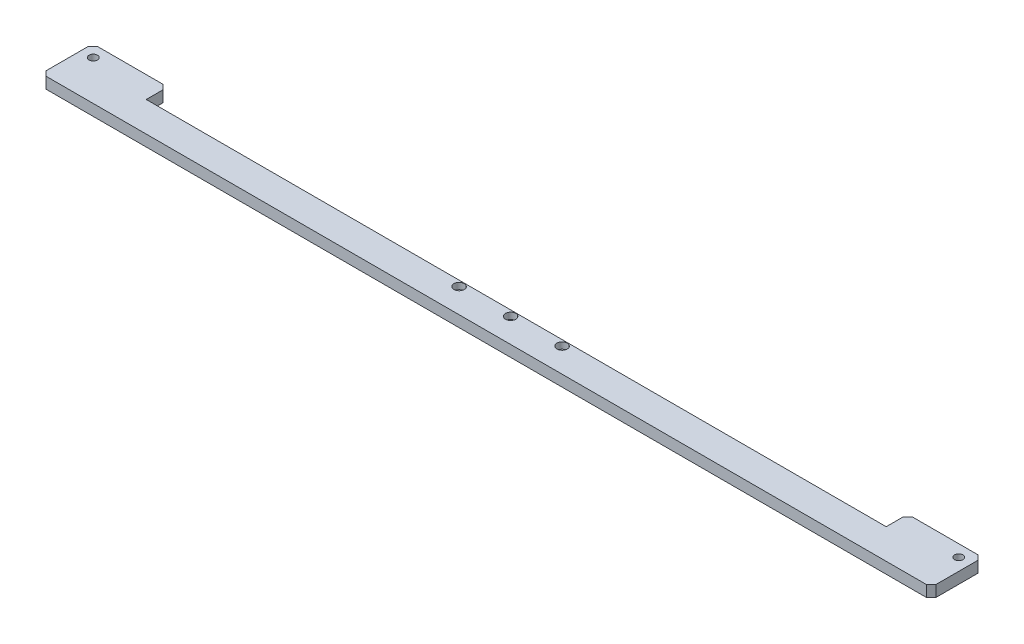
SolidWorks part; units mm, degrees
material "A6061"
ref_plane "前基準面" through (0, 0, 0) normal (0, 0, 1) x (1, 0, 0)
ref_plane "上基準面" through (0, 0, 0) normal (0, 1, 0) x (1, 0, 0)
ref_plane "右基準面" through (0, 0, 0) normal (1, 0, 0) x (0, 0, -1)
sketch "草图1" plane through (0, 0, 0) normal (0, 1, 0) x (1, 0, 0)
  line L1 (-475, -27.5) -> (475, -27.5)
  line L2 (-475, -27.5) -> (-475, 27.5)
  line L3 (-475, 27.5) -> (475, 27.5)
  line L4 (475, -27.5) -> (475, 27.5)
  line L5 (-475, -27.5) -> (475, 27.5) construction
  line L6 (-475, 27.5) -> (475, -27.5) construction
  point P0 (0, 0)
  dimension "D1" = 950
  dimension "D2" = 55
extrude "凸台-拉伸1" add sketch "草图1" along normal mid plane 12
sketch "草图2" plane through (0, 6, 0) normal (0, 1, 0) x (1, 0, 0)
  line L0 (475, 27.5) -> (-475, 27.5) construction
  line L1 (395, 27.5) -> (-395, 27.5)
  line L2 (395, 27.5) -> (395, 4.5)
  line L3 (395, 4.5) -> (-395, 4.5)
  line L4 (-395, 27.5) -> (-395, 4.5)
  line L5 (0, 27.5) -> (0, -27.5) construction
  line L6 (-475, -27.5) -> (475, -27.5) construction
  line L7 (475, -27.5) -> (475, 27.5) construction
  dimension "D1" = 80
  dimension "D2" = 23
extrude "切除-拉伸1" cut sketch "草图2" against normal up to surface (12 mm away) up to face at (0, -6, 0)
chamfer "倒角1" distance 5 angle 45 6 edges at (-475, 0, -27.5) (395, 0, -27.5) (475, 0, -27.5) (-395, 0, -27.5) (-475, 0, 27.5) (475, 0, 27.5)
hole_wizard "M8 间隙孔1" positions "草图3" profile "草图4" hole size "M8" standard "GB" end condition through all
sketch "草图3" plane through (0, -6, 0) normal (0, -1, 0) x (-1, 0, 0)
  line L0 (0, -27.5) -> (0, 88.4483) construction
  line L1 (470, -27.5) -> (-470, -27.5) construction
  line L3 (400, 27.5) -> (470, 27.5) construction
  point P0 (462, 15)
  point P9 (-462, 15)
  dimension "D1" = 924
  dimension "D2" = 12.5
sketch "草图4" plane through (-462, -6, -15) normal (1, 0, 0) x (0, 0, -1)
  line L0 (0, 0) -> (0, 12)
  line L1 (0, 12) -> (4.5, 12)
  line L2 (4.5, 12) -> (4.5, 0)
  line L5 (4.5, 0) -> (0, 0)
  line L11 (0, -6.35) -> (0, 107.95) construction
  dimension "通孔孔直径" = 9
  dimension "通孔孔深度" = 12
hole_wizard "打孔尺寸(%根据)内六角圆柱头螺钉的类型1" positions "草图5" profile "草图6" counterbore size "M6" standard "GB" end condition through all
sketch "草图5" plane through (0, 6, 0) normal (0, 1, 0) x (1, 0, 0)
  line L0 (0, 0) -> (0, -72.0736) construction
  line L2 (-395, 4.5) -> (395, 4.5) construction
  point P0 (55, -1.5)
  point P2 (0, -1.5)
  point P10 (-55, -1.5)
  dimension "D1" = 110
  dimension "D2" = 6
sketch "草图6" plane through (55, 6, 1.5) normal (1, 0, 0) x (0, 0, 1)
  line L0 (0, 0) -> (0, 12)
  line L1 (0, 12) -> (3.3, 12)
  line L3 (3.3, 12) -> (3.3, 6.8)
  line L4 (3.3, 6.8) -> (5.5, 6.8)
  line L5 (5.5, 6.8) -> (5.5, 0)
  line L7 (5.5, 0) -> (0, 0)
  line L11 (0, -6.35) -> (0, 107.95) construction
  dimension "通孔孔直径" = 6.6
  dimension "通孔孔深度" = 12
  dimension "柱形沉头孔直径" = 11
  dimension "柱形沉头孔深度" = 6.8
